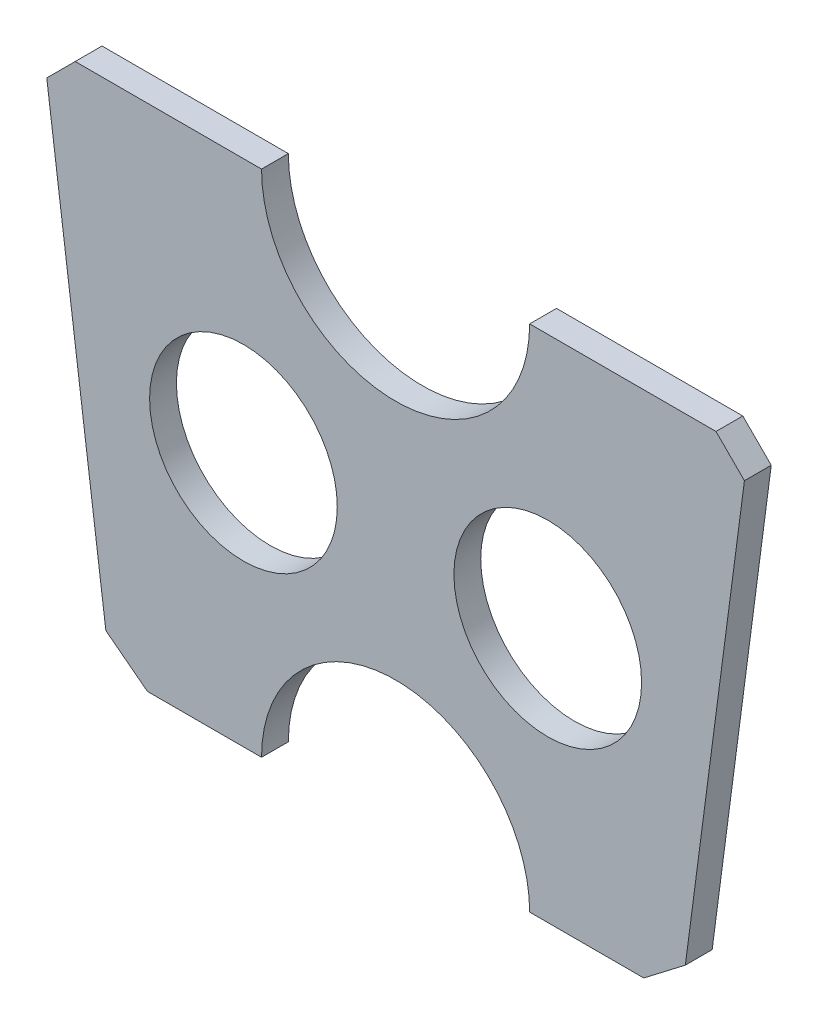
SolidWorks part; units mm, degrees
ref_plane "Front Plane" through (0, 0, 0) normal (0, 0, 1) x (1, 0, 0)
ref_plane "Top Plane" through (0, 0, 0) normal (0, 1, 0) x (1, 0, 0)
ref_plane "Right Plane" through (0, 0, 0) normal (1, 0, 0) x (0, 0, -1)
sketch "Sketch1" plane through (0, 0, 0) normal (0, 0, 1) x (1, 0, 0)
  line L0 (0, -104.3508) -> (0, 101.8828) construction
  line L1 (-48.4994, 0) -> (155.3025, 0) construction
  line L2 (131.5, 101.8828) -> (131.5, -32.0826) construction
  line L3 (106.5, 17.1322) -> (106.5, -104.3508) construction
  line L4 (56.75, 82.1012) -> (56.75, -86.9961) construction
  line L5 (50, 95) -> (119.5, 95)
  line L6 (50, -95) -> (92.5627, -95)
  line L7 (130.1047, 84.3953) -> (108.0655, -83.1025)
  line L8 (119.5, 95) -> (130.1047, 84.3953)
  line L9 (108.0655, -83.1025) -> (92.5627, -95)
  line L10 (-50, -95) -> (-92.5627, -95)
  line L11 (-108.0655, -83.1025) -> (-92.5627, -95)
  line L12 (-119.5, 95) -> (-130.1047, 84.3953)
  line L13 (-130.1047, 84.3953) -> (-108.0655, -83.1025)
  line L14 (-50, 95) -> (-119.5, 95)
  circle A0 centre (56.75, 0) radius 35
  arc A1 (-50, 95) -> (50, 95) centre (0, 95) ccw
  arc A2 (50, -95) -> (-50, -95) centre (0, -95) ccw
  circle A3 centre (-56.75, 0) radius 35
  point P19 (131.5, 95)
  point P20 (106.5, -95)
  point P29 (-106.5, -95)
  dimension "D4" = 70
  dimension "D7" = 100
  dimension "D8" = 100
  dimension "D1" = 131.5
  dimension "D2" = 106.5
  dimension "D3" = 56.75
  dimension "D5" = 95
  dimension "D6" = 95
  dimension "D9" = 12
  dimension "D10" = 45
  dimension "D11" = 12
  dimension "D12" = 45
extrude "Boss-Extrude1" add sketch "Sketch1" along normal blind 10
